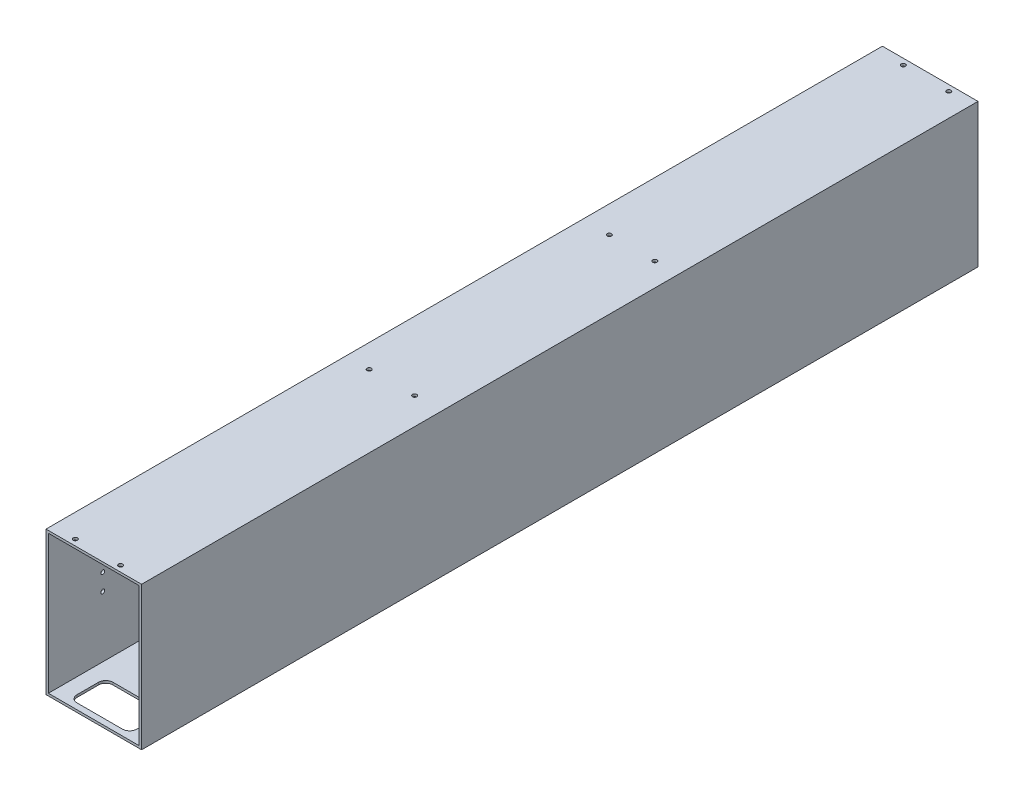
SolidWorks part; units mm, degrees
material "6061Al"
ref_plane "前视基准面" through (0, 0, 0) normal (0, 0, 1) x (1, 0, 0)
ref_plane "上视基准面" through (0, 0, 0) normal (0, 1, 0) x (1, 0, 0)
ref_plane "右视基准面" through (0, 0, 0) normal (1, 0, 0) x (0, 0, -1)
sketch "草图1" plane through (0, 0, 0) normal (0, 0, 1) x (1, 0, 0)
  line L1 (-40, -60) -> (40, -60)
  line L2 (-40, -60) -> (-40, 60)
  line L3 (-40, 60) -> (40, 60)
  line L4 (40, -60) -> (40, 60)
  line L5 (-40, -60) -> (40, 60) construction
  line L6 (-40, 60) -> (40, -60) construction
  point P0 (0, 0)
  dimension "D1" = 80
  dimension "D2" = 120
extrude "拉伸-薄壁1" add sketch "草图1" along normal mid plane 700 thin thin type one direction reverse wall 2
sketch "草图3" plane through (0, 0, 350) normal (0, 0, 1) x (1, 0, 0)
  line L0 (-40, -60) -> (40, -60) construction
  line L1 (-38, -58) -> (38, -58)
  line L2 (-38, -58) -> (-38, -60)
  line L3 (-38, -60) -> (38, -60)
  line L4 (38, -58) -> (38, -60)
  line L6 (38, -58) -> (38, 58) construction
extrude "切除-拉伸1" [suppressed] cut sketch "草图3" against normal through all
sketch "草图4" plane through (-40, 0, 0) normal (-1, 0, 0) x (0, 0, 1)
  line L0 (350, -60) -> (-350, -60) construction
  circle A2 centre (0, -20) radius 25
  dimension "D1" = 50
  dimension "D2" = 40
extrude "切除-拉伸2" cut sketch "草图4" against normal up to next
hole_wizard "M4 螺纹孔1" positions "草图7" profile "草图8" tap size "M4" standard "ISO"
sketch "草图7" plane through (-40, 0, 0) normal (-1, 0, 0) x (0, 0, 1)
  line L0 (0, 0) -> (0, -123.9236) construction
  line L1 (304.5, 15) -> (304.5, -7) construction
  line L2 (-304.5, 15) -> (-304.5, -7) construction
  line L4 (350, 60) -> (-350, 60) construction
  point P0 (304.5, 29)
  point P3 (304.5, 15)
  point P17 (304.5, 7)
  point P18 (304.5, -7)
  point P23 (-304.5, -7)
  point P24 (-304.5, 7)
  point P25 (-304.5, 15)
  point P26 (-304.5, 29)
  dimension "D2" = 22
  dimension "D3" = 304.5
  dimension "D4" = 31
  dimension "D5" = 45
  dimension "D1" = 2
sketch "草图8" plane through (-40, 29, 304.5) normal (0, 1, 0) x (0, 0, 1)
  line L0 (0, 0) -> (0, 2)
  line L1 (0, 2) -> (1.65, 2)
  line L2 (1.65, 2) -> (1.65, 0)
  line L5 (1.65, 0) -> (0, 0)
  line L11 (0, -6.35) -> (0, 107.95) construction
  dimension "通孔螺纹孔钻头直径" = 3.3
  dimension "通孔螺纹孔钻头深度" = 2
cosmetic thread "孔螺蚊线5" parameters "D2"=4
cosmetic thread "孔螺蚊线6" parameters "D2"=4
cosmetic thread "孔螺蚊线7" parameters "D2"=4
cosmetic thread "孔螺蚊线8" parameters "D2"=4
cosmetic thread "孔螺蚊线9" parameters "D2"=4
cosmetic thread "孔螺蚊线10" parameters "D2"=4
cosmetic thread "孔螺蚊线11" parameters "D2"=4
cosmetic thread "孔螺蚊线12" parameters "D2"=4
hole_wizard "M4 间隙孔1" positions "草图9" profile "草图10" hole size "M4" standard "ISO"
sketch "草图9" plane through (0, 60, 0) normal (0, 1, 0) x (1, 0, 0)
  line L1 (0, 0) -> (137.2059, 0) construction
  line L2 (-40, -315) -> (-40, 315) construction
  point P0 (-14.175, 266)
  point P3 (10.825, 266)
  point P6 (-14.175, 166)
  point P9 (10.825, 166)
  point P24 (-10.825, -166)
  point P27 (14.175, -166)
  point P30 (-10.825, -266)
  point P33 (14.175, -266)
  dimension "D1" = 25.825
  dimension "D2" = 29.175
  dimension "D3" = 50.825
  dimension "D4" = 54.175
  dimension "D5" = 166
  dimension "D6" = 266
  dimension "D7" = 166
  dimension "D8" = 266
sketch "草图10" plane through (-14.175, 60, -266) normal (1, 0, 0) x (0, 0, 1)
  line L0 (0, 0) -> (0, 2)
  line L1 (0, 2) -> (2.4, 2)
  line L2 (2.4, 2) -> (2.4, 0)
  line L5 (2.4, 0) -> (0, 0)
  line L11 (0, -6.35) -> (0, 107.95) construction
  dimension "通孔孔直径" = 4.8
  dimension "通孔孔深度" = 2
hole_wizard "M5 间隙孔1" positions "草图11" profile "草图12" hole size "M5" standard "ISO"
sketch "草图11" plane through (-40, 0, 0) normal (-1, 0, 0) x (0, 0, 1)
  point P0 (-266, 53)
  point P3 (-266, -26)
  point P6 (-166, 53)
  point P9 (166, 53)
  point P12 (266, 53)
  point P15 (266, -26)
  dimension "D1" = 166
  dimension "D2" = 266
  dimension "D3" = 166
  dimension "D4" = 266
  dimension "D5" = 53
  dimension "D6" = 26
sketch "草图12" plane through (-40, 53, -266) normal (0, 1, 0) x (0, 0, 1)
  line L0 (0, 0) -> (0, 2)
  line L1 (0, 2) -> (2.9, 2)
  line L2 (2.9, 2) -> (2.9, 0)
  line L5 (2.9, 0) -> (0, 0)
  line L11 (0, -6.35) -> (0, 107.95) construction
  dimension "通孔孔直径" = 5.8
  dimension "通孔孔深度" = 2
hole_wizard "M3 间隙孔1" positions "草图13" profile "草图14" hole size "M3" standard "ISO"
sketch "草图13" plane through (0, 60, 0) normal (0, 1, 0) x (1, 0, 0)
  point P0 (-17.5, 345)
  point P3 (20.5, 345)
  point P6 (20.5, 99)
  point P9 (-17.5, 99)
  point P12 (-20.5, -345)
  point P15 (17.5, -345)
  point P18 (-20.5, -99)
  point P21 (17.5, -99)
sketch "草图14" plane through (-17.5, 60, -345) normal (1, 0, 0) x (0, 0, 1)
  line L0 (0, 0) -> (0, 2)
  line L1 (0, 2) -> (1.8, 2)
  line L2 (1.8, 2) -> (1.8, 0)
  line L5 (1.8, 0) -> (0, 0)
  line L11 (0, -6.35) -> (0, 107.95) construction
  dimension "通孔孔直径" = 3.6
  dimension "通孔孔深度" = 2
other "移动面1" [suppressed] parameters "D1"=5
sketch "草图16" plane through (0, -60, 0) normal (0, -1, 0) x (1, 0, 0)
  line L0 (0, 0) -> (0, 350) construction
  line L1 (-40, 350) -> (40, 350) construction
  line L2 (-25, 330) -> (25, 330) construction
  line L3 (-25, 345) -> (25, 345)
  line L4 (-25, 345) -> (-25, 315)
  line L5 (-25, 315) -> (25, 315)
  line L6 (25, 345) -> (25, 315)
  line L7 (-25.5, 120) -> (25.5, 120) construction
  line L8 (-30, 195) -> (30, 195)
  line L9 (-30, 195) -> (-30, 95)
  line L10 (-30, 95) -> (30, 95)
  line L11 (30, 195) -> (30, 95)
  line L13 (-25.5, 94) -> (-25.5, 350) construction
  line L14 (25.5, 94) -> (25.5, 350) construction
  line L16 (0, 0) -> (111.4, 0) construction
  line L17 (-25.5, -120) -> (25.5, -120) construction
  line L18 (-25, -330) -> (25, -330) construction
  line L19 (30, -195) -> (30, -95)
  line L20 (-30, -95) -> (30, -95)
  line L21 (-30, -195) -> (-30, -95)
  line L22 (-30, -195) -> (30, -195)
  line L23 (25, -345) -> (25, -315)
  line L24 (-25, -315) -> (25, -315)
  line L25 (-25, -345) -> (-25, -315)
  line L26 (-25, -345) -> (25, -345)
  dimension "D1" = 50
  dimension "D2" = 30
  dimension "D3" = 20
  dimension "D4" = 60
  dimension "D5" = 120
  dimension "D6" = 100
  dimension "D7" = 25
extrude "切除-拉伸3" cut sketch "草图16" against normal up to next
fillet "圆角1" radius 6 16 edges at (25, -59, -345) (-25, -59, -345) (-25, -59, -315) (25, -59, -315) (30, -59, -195) (-30, -59, -195) (30, -59, -95) (-30, -59, 95) (-30, -59, 195) (30, -59, 195) (30, -59, 95) (-25, -59, 315) (-25, -59, 345) (25, -59, 345) (25, -59, 315) (-30, -59, -95)
